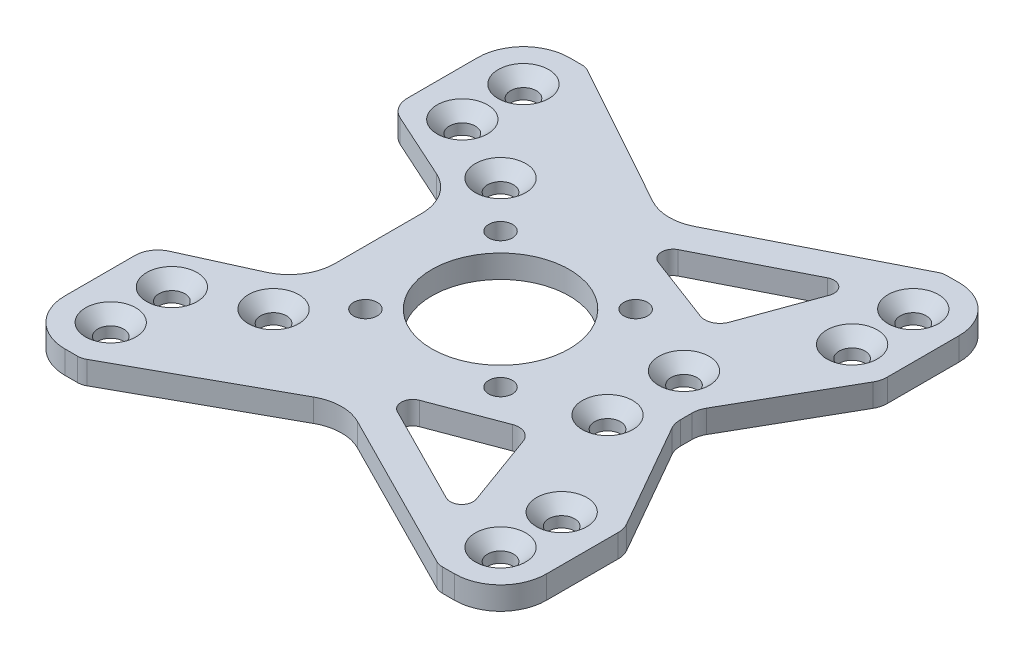
SolidWorks part; units mm, degrees
material "Thornel Mat VMA"
ref_plane "前视基准面" through (0, 0, 0) normal (0, 0, 1) x (1, 0, 0)
ref_plane "上视基准面" through (0, 0, 0) normal (0, 1, 0) x (1, 0, 0)
ref_plane "右视基准面" through (0, 0, 0) normal (1, 0, 0) x (0, 0, -1)
other "Configuration Table"
sketch "草图1" plane through (0, 0, 0) normal (0, 1, 0) x (1, 0, 0)
  line L0 (0, 0) -> (0, 12.5) construction
  line L1 (-33, 33) -> (33, 33)
  line L2 (-33, 33) -> (-33, -33)
  line L3 (-33, -33) -> (33, -33)
  line L4 (33, 33) -> (33, -33)
  line L5 (-33, 33) -> (33, -33) construction
  line L6 (-33, -33) -> (33, 33) construction
  line L7 (0, 0) -> (43.9775, 0) construction
  line L8 (0, 0) -> (0, 20.2995) construction
  line L9 (-24, 27) -> (-24, 19) construction
  line L10 (-24, 27) -> (27, 27) construction
  circle A0 centre (0, 0) radius 12.5 construction
  circle A5 centre (0, 0) radius 9
  circle A6 centre (-24, 19) radius 1.55
  circle A7 centre (-24, 27) radius 1.55
  circle A8 centre (-24, -19) radius 1.55
  circle A9 centre (-24, -27) radius 1.55
  circle A14 centre (-14.8492, 14.8492) radius 1.55
  circle A15 centre (19, 5) radius 1.55
  circle A16 centre (19, -5) radius 1.55
  circle A17 centre (-14.8492, -14.8492) radius 1.55
  circle A18 centre (8.8388, 8.8388) radius 1.55
  circle A19 centre (8.8388, -8.8388) radius 1.55
  circle A20 centre (-8.8388, -8.8388) radius 1.55
  circle A21 centre (-8.8388, 8.8388) radius 1.55
  circle A22 centre (27, 27) radius 1.55
  circle A23 centre (27, 19) radius 1.55
  circle A24 centre (27, -19) radius 1.55
  circle A25 centre (27, -27) radius 1.55
  point P18 (0, 0)
  point P49 (0, 0)
  dimension "D1" = 25
  dimension "D4" = 3.1
  dimension "D6" = 18
  dimension "D8" = 3.1
  dimension "D9" = 19
  dimension "D10" = 24
  dimension "D11" = 21
  dimension "D12" = 5
  dimension "D2" = 66
  dimension "D3" = 66
  dimension "D7" = 8
  dimension "D13" = 19
  dimension "D15" = 51
  dimension "D14" = 2
  dimension "D5" = 4
extrude "凸台-拉伸1" add sketch "草图1" along normal blind 3
hole_wizard "M3 十字槽半沉头木螺钉的锥形沉头孔1" positions "草图7" profile "草图3" countersink size "M3" standard "GB"
sketch "草图7" plane through (0, 3, 0) normal (0, 1, 0) x (1, 0, 0)
  point P0 (-24, 27)
  point P3 (-24, 19)
  point P6 (-24, -19)
  point P9 (-24, -27)
  point P24 (-14.8492, 14.8492)
  point P27 (-14.8492, -14.8492)
  point P30 (19, -5)
  point P33 (19, 5)
  point P41 (27, 19)
  point P44 (27, 27)
  point P47 (27, -19)
  point P50 (27, -27)
sketch "草图3" plane through (-24, 3, -27) normal (1, 0, 0) x (0, 0, 1)
  line L0 (0, 0) -> (0, 8.5215)
  line L1 (0, 8.5215) -> (1.7, 7.5)
  line L2 (1.7, 7.5) -> (1.7, 1.6)
  line L3 (1.7, 1.6) -> (3.3, 0)
  line L5 (3.3, 0) -> (0, 0)
  line L6 (-1.7, 1.6) -> (-3.3, 0) construction
  line L10 (0, 8.5215) -> (-1.7, 7.5) construction
  line L11 (0, -6.35) -> (0, 107.95) construction
  dimension "孔直径" = 3.4
  dimension "孔深度" = 7.5
  dimension "近端锥形沉头孔直径" = 6.6
  dimension "近端锥形沉头孔角度" = 90
  dimension "导头角度" = 118
sketch "草图8" plane through (0, 3, 0) normal (0, 1, 0) x (1, 0, 0)
  line L0 (-33, -33) -> (33, -33) construction
  line L1 (-33, 33) -> (-30, 33)
  line L2 (-33, 33) -> (-33, -33)
  line L3 (-33, -33) -> (-30, -33)
  line L4 (-30, 33) -> (-30, -33)
  dimension "D1" = 3
extrude "切除-拉伸3" cut sketch "草图8" against normal through all and the other way through all
fillet "圆角1" radius 6 4 edges at (33, 1.5, 33) (33, 1.5, -33) (-30, 1.5, 33) (-30, 1.5, -33)
sketch "草图5" plane through (0, 3, 0) normal (0, 1, 0) x (1, 0, 0)
  line L0 (-24, 19) -> (-14.8492, 14.8492) construction
  line L1 (-30, -27) -> (-30, 27) construction
  line L2 (-31, 16.3554) -> (-31, -16.3554)
  line L3 (-31, -16.3554) -> (-16, -9.5515)
  line L4 (-16, -9.5515) -> (-16, 9.5515)
  line L5 (-16, 9.5515) -> (-31, 16.3554)
  line L6 (0, 0) -> (3.6093, 0) construction
  line L7 (0, 0) -> (0, 4.6016) construction
  line L9 (27, 19) -> (19, 5) construction
  line L10 (34, 18.5519) -> (24.3, 1.5769)
  line L12 (24.3, 1.5769) -> (24.3, -1.5769)
  line L13 (24.3, -1.5769) -> (34, -18.5519)
  line L14 (34, -18.5519) -> (34, 18.5519)
  line L15 (33, -27) -> (33, 27) construction
  line L16 (27, 27) -> (-8.8388, 8.8388) construction
  line L17 (-23.6397, 34) -> (26.8762, 34)
  line L18 (26.8762, 34) -> (0.5149, 20.6415)
  line L19 (0.5149, 20.6415) -> (-23.6397, 34)
  line L20 (27, 33) -> (-24, 33) construction
  line L21 (-24, 27) -> (8.8388, 8.8388) construction
  line L22 (21.2359, 26.6575) -> (1.839, 16.8282)
  line L23 (1.839, 16.8282) -> (15.7505, 11.5726)
  line L24 (15.7505, 11.5726) -> (21.2359, 26.6575)
  line L25 (27, 27) -> (19, 5) construction
  line L26 (19, 5) -> (8.8388, 8.8388) construction
  line L27 (1.839, -16.8282) -> (15.7505, -11.5726)
  line L28 (15.7505, -11.5726) -> (21.2359, -26.6575)
  line L29 (21.2359, -26.6575) -> (1.839, -16.8282)
  line L30 (26.8762, -34) -> (0.5149, -20.6415)
  line L31 (0.5149, -20.6415) -> (-23.6397, -34)
  line L32 (-23.6397, -34) -> (26.8762, -34)
  circle A0 centre (27, 27) radius 1.7 construction
  circle A1 centre (0, 0) radius 9 construction
  circle A2 centre (19, 5) radius 1.7 construction
  circle A3 centre (27, 19) radius 1.7 construction
  dimension "D2" = 5.3
  dimension "D3" = 16
  dimension "D4" = 1
  dimension "D5" = 5.3
  dimension "D6" = 6.3
  dimension "D7" = 1
  dimension "D8" = 6.3
  dimension "D9" = 6.3
  dimension "D10" = 4
  dimension "D11" = 5.3
  dimension "D12" = 5
  dimension "D13" = 1
extrude "切除-拉伸2" cut sketch "草图5" against normal through all
fillet "圆角2" radius 2 6 edges at (15.7505, 1.5, 11.5726) (15.7505, 1.5, -11.5726) (24.9028, 1.5, -33) (-21.8315, 1.5, -33) (24.9028, 1.5, 33) (-21.8315, 1.5, 33)
fillet "圆角3" radius 1.5 4 edges at (21.2359, 1.5, -26.6575) (1.839, 1.5, -16.8282) (1.839, 1.5, 16.8282) (21.2359, 1.5, 26.6575)
fillet "圆角4" radius 6 4 edges at (-16, 1.5, -9.5515) (-16, 1.5, 9.5515) (0.5149, 1.5, -20.6415) (0.5149, 1.5, 20.6415)
fillet "圆角5" radius 3 6 edges at (33, 1.5, -16.8019) (33, 1.5, 16.8019) (24.3, 1.5, -1.5769) (24.3, 1.5, 1.5769) (-30, 1.5, 15.9018) (-30, 1.5, -15.9018)
